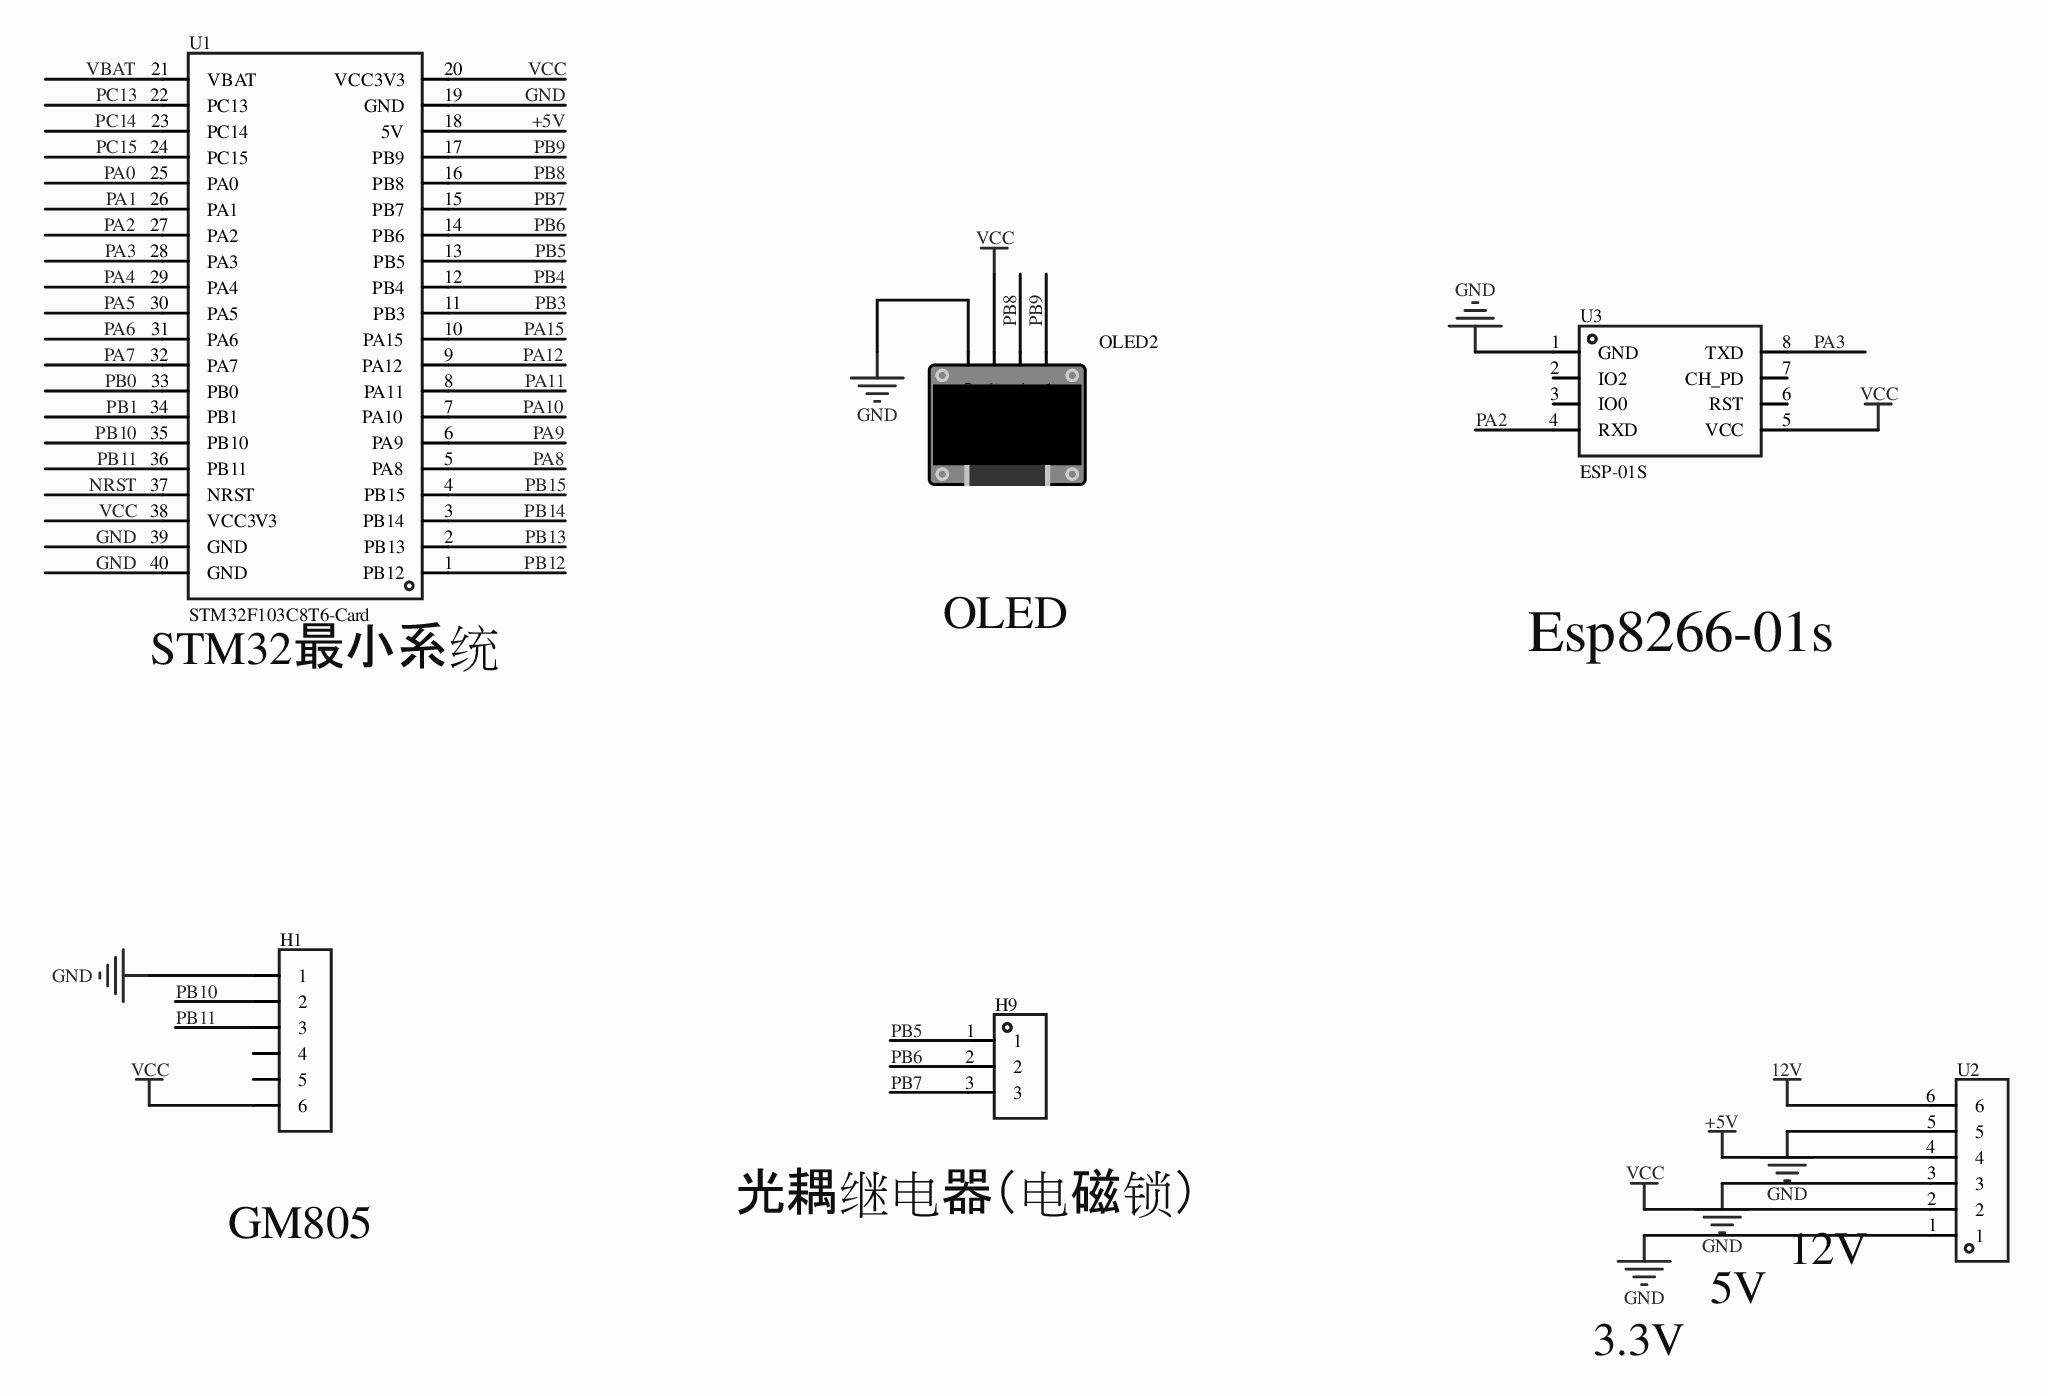
[diagram p0: MISC52106-3.schdoc]
# Altium project MISC52106-2.PrjPcb
1 sheet, 6 parts. Net scope: global (net labels, ports and power ports of the same name join across sheets).
Board file: MISC52106.pcbdoc

## Sheet MISC52106-3.schdoc
size 297 x 209 mm; Version: V1.0; @Project Name: MISC52106; @Page Count: 1; @Update Date: 2026-05-02; @Create Date: 2026-05-02; @Schematic Name: MISC52106; @Page No: 1; @Create Time: 23:22:16; @Update Time: 17:32:40; @Board Name: MISC52106

### Parts
H1  (no value)  [HDR-TH_6P-P2.54-V-M-1]
H9  (no value)  [HDR-TH_3P-P2.54-V-F]
OLED2  (no value)  [0.96OLED_4P]
U1  STM32F103C8T6-Card  [CONN-TH_L53.3-W22.9_STM32F103C8T6-CARD]
U2  LG128V 5.08 6P180度螺丝用十字带一字型  [CONN-TH_6P-P5.00_LG128V]  (value not drawn)
U3  ESP-01S  [WIFIM-TH_ESP-01S]

### Nets
12V: U2.6
+5V: U1.18(5V) U2.4
GND: H1.1 OLED2.1(GND) U1.19(GND) U1.39(GND) U1.40(GND) U2.1 U2.3 U2.5 U3.1(GND)
VCC: H1.6 OLED2.2(VCC) U1.20(VCC3V3) U1.38(VCC3V3) U2.2 U3.5(VCC)
NRST: U1.37(NRST)
PA0: U1.25(PA0)
PA1: U1.26(PA1)
PA2: U1.27(PA2) U3.4(RXD)
PA3: U1.28(PA3) U3.8(TXD)
PA4: U1.29(PA4)
PA5: U1.30(PA5)
PA6: U1.31(PA6)
PA7: U1.32(PA7)
PA8: U1.5(PA8)
PA9: U1.6(PA9)
PA10: U1.7(PA10)
PA11: U1.8(PA11)
PA12: U1.9(PA12)
PA15: U1.10(PA15)
PB0: U1.33(PB0)
PB1: U1.34(PB1)
PB3: U1.11(PB3)
PB4: U1.12(PB4)
PB5: H9.1 U1.13(PB5)
PB6: H9.2 U1.14(PB6)
PB7: H9.3 U1.15(PB7)
PB8: OLED2.3(SCL) U1.16(PB8)
PB9: OLED2.4(SDA) U1.17(PB9)
PB10: H1.2 U1.35(PB10)
PB11: H1.3 U1.36(PB11)
PB12: U1.1(PB12)
PB13: U1.2(PB13)
PB14: U1.3(PB14)
PB15: U1.4(PB15)
PC13: U1.22(PC13)
PC14: U1.23(PC14)
PC15: U1.24(PC15)
VBAT: U1.21(VBAT)

Not connected (* = marked no-connect by the designer): H1 4 5; U3 2(IO2)* 3(IO0)* 6(RST)* 7(CH_PD)*

### Notes on the sheet
- 硬件有stm32，
  电源模块，
  oled,
  esp8266,
  gm805;
  1路光耦继电器驱动模块;
  电磁锁。
  OLED的scl, sda接stm的pb1,pb0;
  esp的rxtx接pa3,pa2
  ;gm805的txrx接pb10，pb11，
  电源接电源模块的5v;
  继电器单片机端接pb5，pb6，pb7，
  供电口是电源模块的12v，
  电磁锁接继电器输出端
- OLED
- (near U1) STM32最小系统
- Esp8266-01s
- (near H1) GM805
- (near H9) 光耦继电器（电磁锁）
- (near U2) 12V
- 3.3V
- 5V

### Library data of the parts
H1 = HDR-M_2.54_1x6P: Symbol: Header-Male-2.54_1x6; ConvertToPcb: yes; ModelId: 60739dffc9b04830a286435b0fefbd4a0819f05c4eef4c71ace90d822a990e87; ModelName: HDR2.54-M-LI-1X6P; ModelTransform: 599.999,100,0,0,0,0,0,0,-118.11; Device: HDR-M_2.54_1x6P; AddInBom: yes; SupplierPart: C37208; Supplier Footprint: 插件; FootprintName: HDR-TH_6P-P2.54-V-M-1
H9 = HDR-F_2.54_1x3P: Symbol: PM254V-11-03-H85; ConvertToPcb: yes; ModelId: f3b3cc5aae9641bf9e56fc160cef875b; ModelName: HDR2.54-F-LI-1X3P; ModelTransform: 299.9994,100,0,0,0,0,0,0,-118.11; Device: HDR-F_2.54_1x3P; AddInBom: yes; SupplierPart: C541850; Supplier Footprint: 插件; FootprintName: HDR-TH_3P-P2.54-V-F
OLED2 = 0.96OLED模块_4P: ConvertToPcb: yes; ModelId: 79c000fdb68d45a296c2e9bedf4f9055; ModelTransform: 1393.69792,1318.895,0,0,0,0,0,-560.079,-137.795; Symbol: 0.96OLED模块_4P; Device: 0.96OLED模块_4P; AddInBom: yes; FootprintName: 0.96OLED_4P; Supplier Footprint: 插件; ModelName: 0.96OLED_4P
U1 = STM32F103C8T6-Card: AddInBom: yes; Device: STM32F103C8T6-Card; Symbol: STM32F103C8T6-CARD; FootprintName: CONN-TH_L53.3-W22.9_STM32F103C8T6-CARD; LCSC Part Name: STM32F103C8T6-Card; SupplierPart: C9900077949; ManufacturerPart: STM32F103C8T6-Card; Supplier Footprint: 插件; Supplier: LCSC; ConvertToPcb: yes
U2 = LG128V 5.08 6P180度螺丝用十字带一字型: AddInBom: yes; ModelId: 684ac4b28bf8492ba94907e15d3a15430819f05c4eef4c71ace90d822a990e87; ModelTransform: 1205.5094,393.7,0,0,0,0,-11.811,0,-157.48; Symbol: LG128V 5.08 6P180度螺丝用十字带一字型; Device: LG128V 5.08 6P180度螺丝用十字带一字型; LCSC Part Name: LG128V 5.08 6P180度螺丝用十字带一字型; SupplierPart: C9900009359; ManufacturerPart: LG128V 5.08 6P180度螺丝用十字带一字型; Supplier Footprint: LG128V 5.08 6P180度; JLCPCB Part Class: Extended Part; Supplier: LCSC; ConvertToPcb: yes; FootprintName: CONN-TH_6P-P5.00_LG128V; ModelName: CONN-TH_6P-P5.00_LG128V
U3 = ESP-01S_C111009: 3D Model: eb7175da78ae48b3b1568cfe3027405f0819f05c4eef4c71ace90d822a990e87; 3D Model Transform: 582.676,976.37608,0,0,0,0,0,388.346,-118.11; AddInBom: yes; Symbol: ESP-01S; Device: ESP-01S_C111009; LCSC Part Name: ESP-01S; Supplier Part: C111009; Manufacturer Part: ESP-01S; Supplier Footprint: -; JLCPCB Part Class: Extended Part; Supplier: LCSC; ConvertToPcb: yes; FootprintName: WIFIM-TH_ESP-01S; ModelName: WIFIM-TH_ESP-01S